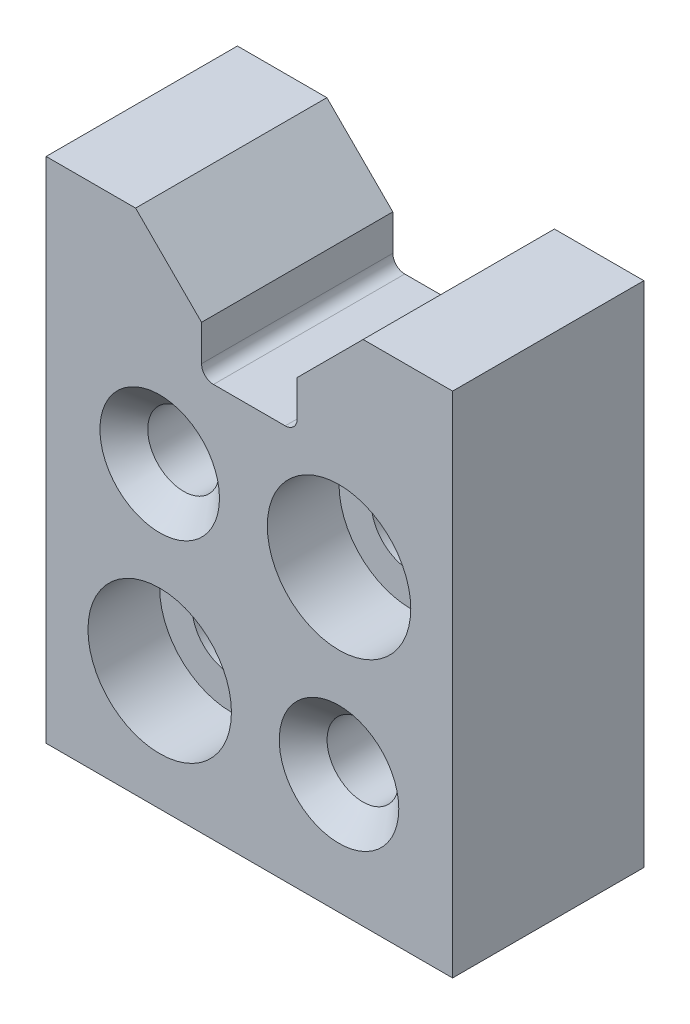
from build123d import *

# Parameters (mm, degrees)
SKETCH1_W                                = 34
SKETCH1_H                                = 45
BASE_EXTRUDE_DEPTH                       = 16
CUT_EXTRUDE1_DEPTH                       = 56.951622292
CBORE_FOR_M5_HEX_HEAD_SCREW1_D           = 6.6
CBORE_FOR_M5_HEX_HEAD_SCREW1_CBORE_D     = 12
CBORE_FOR_M5_HEX_HEAD_SCREW1_CBORE_DEPTH = 6
SKETCH3_R                                = 3
CUT_EXTRUDE4_DEPTH                       = 25
CHAMFER3_SIZE                            = 2
CHAMFER4_SIZE                            = 2
CBORE_FOR_M5_HEX_HEAD_SCREW2_D           = 6.6
CBORE_FOR_M5_HEX_HEAD_SCREW2_CBORE_D     = 12
CBORE_FOR_M5_HEX_HEAD_SCREW2_CBORE_DEPTH = 6
FILLET1_R                                = 1
FILLET2_R                                = 1
SKETCH13_W                               = 37.795873191
SKETCH13_H                               = 5.669380978
CUT_EXTRUDE5_DEPTH                       = 56.951622292


with BuildPart() as part:
    # Sketch1 → Base-Extrude (new body)
    with BuildSketch(Plane.XY):
        with Locations((0, 28.348638498)):
            Rectangle(SKETCH1_W, SKETCH1_H)
    extrude(amount=BASE_EXTRUDE_DEPTH)

    # Sketch2 → Cut-Extrude1 (cut, through all)
    with BuildSketch(Plane.XY.offset(16)):
        Polygon((-4, 38.848638498), (4, 38.848638498), (4, 42.848638498), (12, 50.848638498), (-12, 50.848638498), (-4, 42.848638498), align=None)
    extrude(amount=-CUT_EXTRUDE1_DEPTH, mode=Mode.SUBTRACT)

    # CBORE for M5 Hex Head Screw1 (through all)
    with Locations(Plane.XY.offset(16)):
        with Locations((7.5, 30.848638498)):
            CounterBoreHole(CBORE_FOR_M5_HEX_HEAD_SCREW1_D / 2, CBORE_FOR_M5_HEX_HEAD_SCREW1_CBORE_D / 2, CBORE_FOR_M5_HEX_HEAD_SCREW1_CBORE_DEPTH)

    # Sketch3 → Cut-Extrude4 (cut)
    with BuildSketch(Plane.XY.offset(16)):
        with Locations((-7.5, 30.848638498)):
            Circle(SKETCH3_R)
        with Locations((7.5, 15.848638498)):
            Circle(SKETCH3_R)
    extrude(amount=-CUT_EXTRUDE4_DEPTH, mode=Mode.SUBTRACT)

    # Chamfer3
    chamfer3_edges = [part.edges().sort_by_distance(p)[0] for p in [
        (-10.5, 30.848638498, 16),
        (4.5, 15.848638498, 16),
    ]]
    chamfer(chamfer3_edges, length=CHAMFER3_SIZE)

    # Chamfer4
    chamfer4_edges = [part.edges().sort_by_distance(p)[0] for p in [
        (-10.5, 30.848638498, 0),
        (4.5, 15.848638498, 0),
    ]]
    chamfer(chamfer4_edges, length=CHAMFER4_SIZE)

    # CBORE for M5 Hex Head Screw2 (through all)
    with Locations(Plane.XY.offset(16)):
        with Locations((-7.5, 15.848638498)):
            CounterBoreHole(CBORE_FOR_M5_HEX_HEAD_SCREW2_D / 2, CBORE_FOR_M5_HEX_HEAD_SCREW2_CBORE_D / 2, CBORE_FOR_M5_HEX_HEAD_SCREW2_CBORE_DEPTH)

    # Fillet1
    fillet1_edges = [part.edges().sort_by_distance(p)[0] for p in [
        (-4, 38.848638498, 8),
    ]]
    fillet(fillet1_edges, radius=FILLET1_R)

    # Fillet2
    fillet2_edges = [part.edges().sort_by_distance(p)[0] for p in [
        (4, 38.848638498, 8),
    ]]
    fillet(fillet2_edges, radius=FILLET2_R)

    # Sketch13 → Cut-Extrude5 (cut, through all)
    with BuildSketch(Plane.XY.offset(16)):
        with Locations((-0.227198085, 51.199908502)):
            Rectangle(SKETCH13_W, SKETCH13_H)
    extrude(amount=-CUT_EXTRUDE5_DEPTH, mode=Mode.SUBTRACT)


solid = part.part
